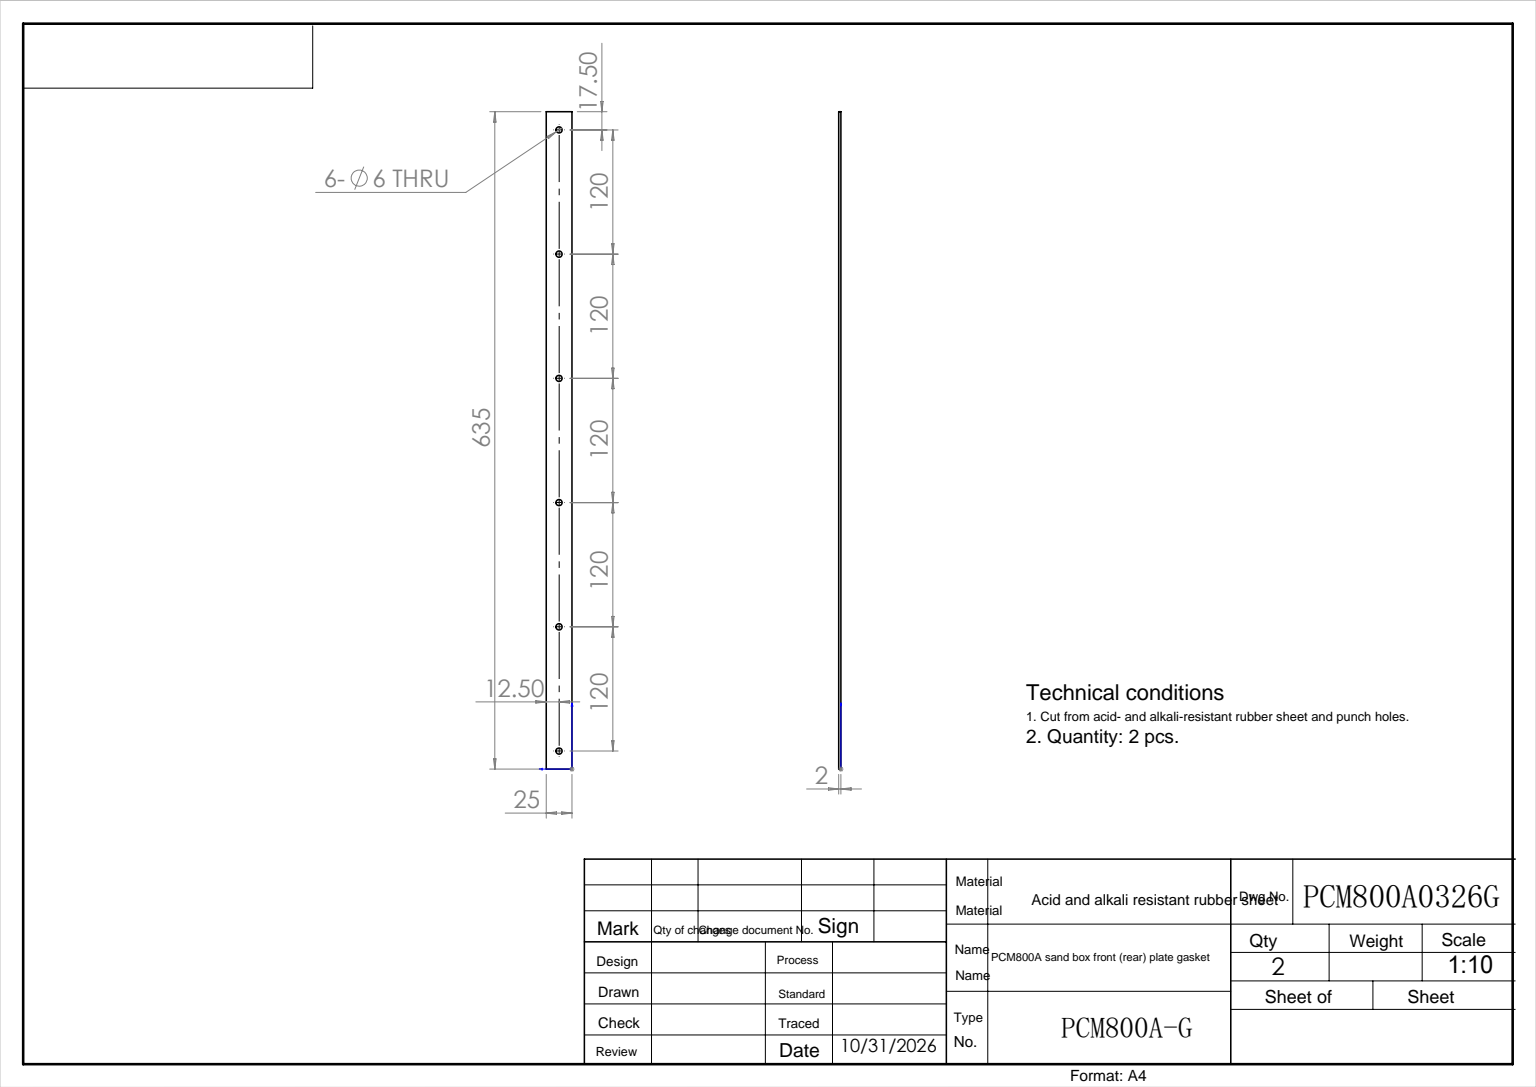
SolidWorks part; units mm, degrees
ref_plane "前视" through (0, 0, 0) normal (0, 0, 1) x (1, 0, 0)
ref_plane "上视" through (0, 0, 0) normal (0, 1, 0) x (1, 0, 0)
ref_plane "右视" through (0, 0, 0) normal (1, 0, 0) x (0, 0, -1)
sketch "草图1" plane through (0, 0, 0) normal (0, 0, 1) x (1, 0, 0)
  line L1 (0, 0) -> (25, 0)
  line L2 (0, 0) -> (0, 635)
  line L3 (0, 635) -> (25, 635)
  line L4 (25, 0) -> (25, 635)
  dimension "D1" = 25
  dimension "D2" = 635
extrude "拉伸1" add sketch "草图1" along normal blind 2
sketch "草图3" plane through (0, 0, 2) normal (0, 0, 1) x (1, 0, 0)
  line L0 (12.5, 635) -> (12.5, 0) construction
  line L1 (25, 635) -> (0, 635) construction
  line L2 (0, 0) -> (25, 0) construction
  line L3 (12.5, 617.5) -> (25, 617.5) construction
  line L4 (25, 0) -> (25, 635) construction
  circle A0 centre (12.5, 617.5) radius 3
  dimension "D1" = 17.5
extrude "切除-拉伸1" cut sketch "草图3" against normal through all
pattern_linear "阵列(线性)1" count 6 spacing 120 along (0, -1, 0) of "切除-拉伸1"
